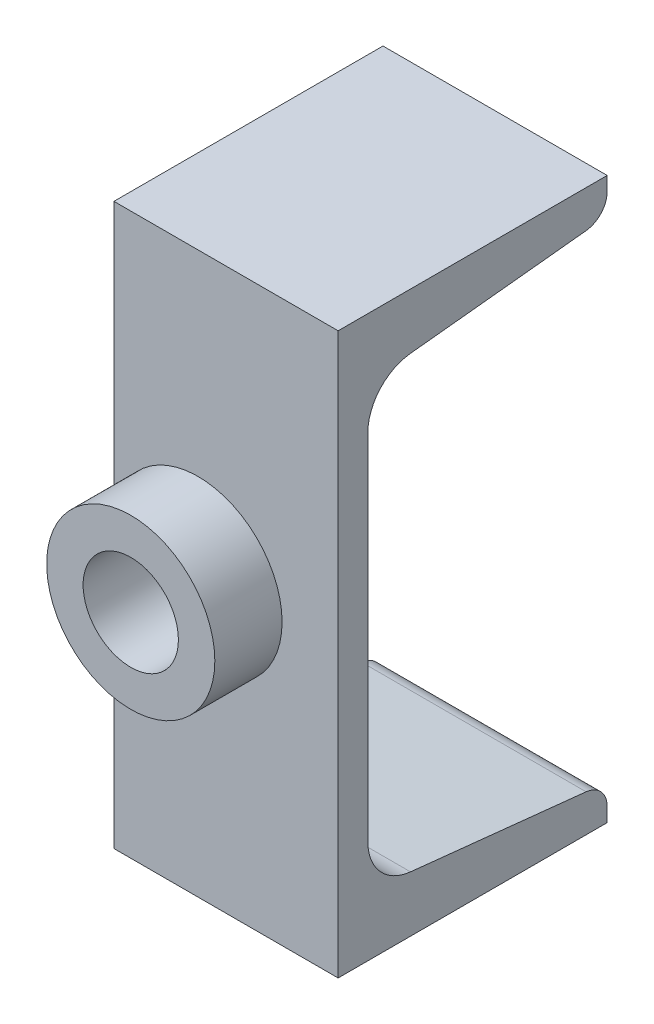
from build123d import *

# Parameters (mm, degrees)
HOT_ROLLED_CHANNEL_GB_T706_2008_10_1_DEPTH = 40
SKETCH2_R                                  = 8.5
CUT_EXTRUDE1_DEPTH                         = 10
SKETCH3_R                                  = 15
SKETCH3_R_2                                = 8.5
BOSS_EXTRUDE1_DEPTH                        = 12


with BuildPart() as part:
    # Sketch1 → Hot-rolled channel gb∕t706-2008 10(1) (new body)
    with BuildSketch(Plane(origin=(0, 0, 0), x_dir=(0, 0, -1), z_dir=(1, 0, 0))):
        with BuildLine():
            Line((48, 100), (0, 100))
            Line((0, 100), (0, 0))
            Line((0, 0), (48, 0))
            Line((48, 0), (48, 2.474327591))
            ThreePointArc((48, 2.474327591), (46.921208267, 5.284676138), (44.239019546, 6.651319552))
            Line((44.239019546, 6.651319552), (12.911508062, 9.943973689))
            ThreePointArc((12.911508062, 9.943973689), (7.483268983, 12.709799645), (5.3, 18.397409799))
            Line((5.3, 18.397409799), (5.3, 81.602590201))
            ThreePointArc((5.3, 81.602590201), (7.483268983, 87.290200355), (12.911508062, 90.056026311))
            Line((12.911508062, 90.056026311), (44.239019546, 93.348680448))
            ThreePointArc((44.239019546, 93.348680448), (46.921208267, 94.715323862), (48, 97.525672409))
            Line((48, 97.525672409), (48, 100))
        make_face()
    extrude(amount=HOT_ROLLED_CHANNEL_GB_T706_2008_10_1_DEPTH)

    # Sketch2 → Cut-Extrude1 (cut)
    with BuildSketch(Plane.XY):
        with Locations((15, 50)):
            Circle(SKETCH2_R)
    extrude(amount=-CUT_EXTRUDE1_DEPTH, mode=Mode.SUBTRACT)


with BuildPart() as body_2:
    # Sketch3 → Boss-Extrude1 (new body)
    with BuildSketch(Plane.XY):
        with Locations((15, 50)):
            Circle(SKETCH3_R)
        with Locations((15, 50)):
            Circle(SKETCH3_R_2, mode=Mode.SUBTRACT)
    extrude(amount=BOSS_EXTRUDE1_DEPTH)


solid = Compound([part.part, body_2.part])
